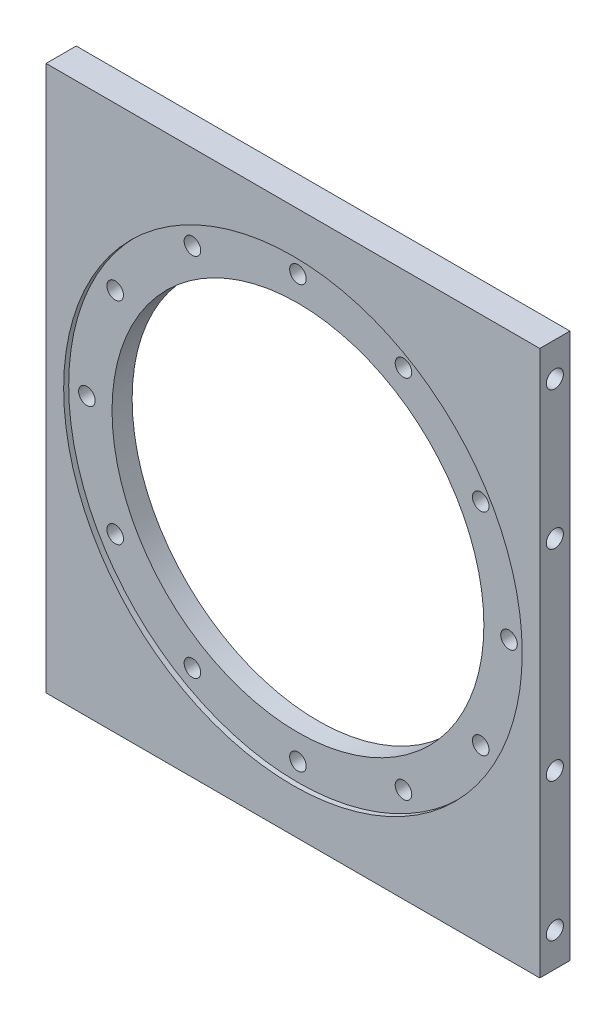
from build123d import *

# Parameters (mm, degrees)
SKETCH_1_W             = 196.5
SKETCH_1_H             = 217
SKETCH_1_R             = 74
EXTRUDE_1_DEPTH        = 12
SKETCH_2_R             = 91.25
CUT_EXTRUDE_1_DEPTH    = 2
CUT_EXTRUDE_START      = -2
SKETCH_3_R             = 91.25
CUT_EXTRUDE_2_DEPTH    = 2
HOLE_WIZARD_M6_1_D     = 6.6
HOLE_WIZARD_M8_1_D     = 6.8
HOLE_WIZARD_M8_1_DEPTH = 19.75
HOLE_WIZARD_M8_1_TIP   = 2.042926105
HOLE_WIZARD_M8_2_D     = 6.8
HOLE_WIZARD_M8_2_DEPTH = 19.75
HOLE_WIZARD_M8_2_TIP   = 2.042926105


with BuildPart() as part:
    # 草图1 → 凸台-拉伸1 (new body)
    with BuildSketch(Plane.XY):
        Rectangle(SKETCH_1_W, SKETCH_1_H)
        Circle(SKETCH_1_R, mode=Mode.SUBTRACT)
    extrude(amount=EXTRUDE_1_DEPTH)

    # 草图2 → 切除-拉伸1 (cut)
    with BuildSketch(Plane(origin=(0, 0, 0), x_dir=(-1, 0, 0), z_dir=(0, 0, -1))):
        Circle(SKETCH_2_R)
    extrude(amount=-CUT_EXTRUDE_1_DEPTH, mode=Mode.SUBTRACT)

    # 草图3 → 切除-拉伸2 (cut)
    with BuildSketch(Plane.XY.offset(12).offset(CUT_EXTRUDE_START)):
        with Locations(Location((0, 0, 0), (0, 0, 180))):
            Circle(SKETCH_3_R)
    extrude(amount=CUT_EXTRUDE_2_DEPTH, mode=Mode.SUBTRACT)

    # M6 间隙孔1 (through all)
    with Locations(Plane.XY.offset(10)):
        with Locations((0, 84), (42, 72.746133918), (72.746133918, 42), (84, 0), (72.746133918, -42), (42, -72.746133918), (0, -84), (-42, -72.746133918), (-72.746133918, -42), (-84, 0), (-72.746133918, 42), (-42, 72.746133918)):
            Hole(HOLE_WIZARD_M6_1_D / 2)

    # M8 螺纹孔1
    with Locations(Plane.ZY.offset(98.25)):
        with Locations((6, 95), (6, 40), (6, -40), (6, -95)):
            Hole(HOLE_WIZARD_M8_1_D / 2, depth=HOLE_WIZARD_M8_1_DEPTH)
            with Locations((0, 0, -(HOLE_WIZARD_M8_1_DEPTH + HOLE_WIZARD_M8_1_TIP / 2))):  # 118° drill point
                Cone(0, HOLE_WIZARD_M8_1_D / 2, HOLE_WIZARD_M8_1_TIP, mode=Mode.SUBTRACT)

    # M8 螺纹孔2
    with Locations(Plane(origin=(98.25, 0, 0), x_dir=(0, 0, -1), z_dir=(1, 0, 0))):
        with Locations((-6, 95), (-6, 40), (-6, -40), (-6, -95)):
            Hole(HOLE_WIZARD_M8_2_D / 2, depth=HOLE_WIZARD_M8_2_DEPTH)
            with Locations((0, 0, -(HOLE_WIZARD_M8_2_DEPTH + HOLE_WIZARD_M8_2_TIP / 2))):  # 118° drill point
                Cone(0, HOLE_WIZARD_M8_2_D / 2, HOLE_WIZARD_M8_2_TIP, mode=Mode.SUBTRACT)


solid = part.part
